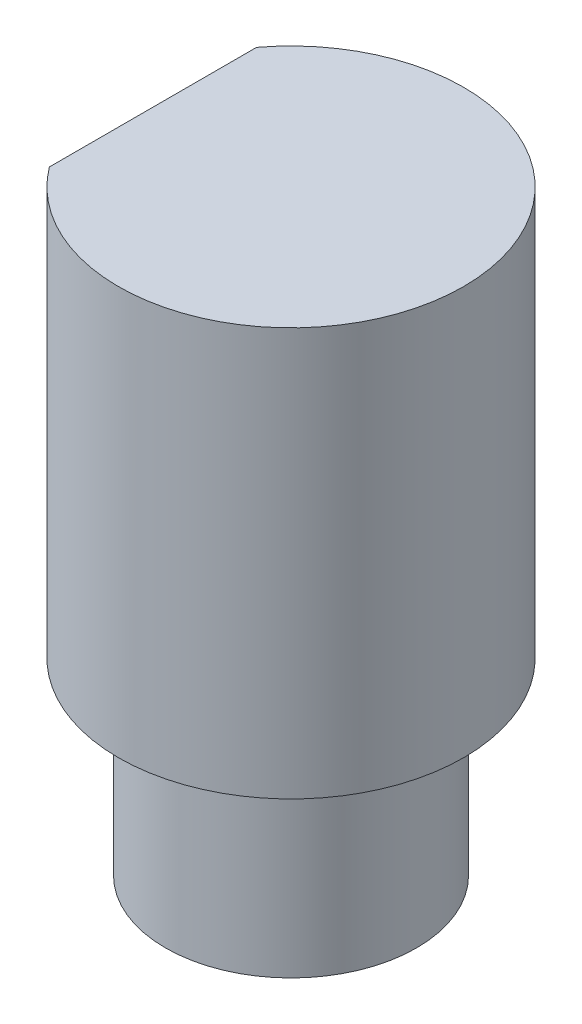
from build123d import *

# Parameters (mm, degrees)
SKETCH1_R           = 20
BOSS_EXTRUDE1_DEPTH = 30
SKETCH2_R           = 27.5
BOSS_EXTRUDE2_DEPTH = 65
CUT_EXTRUDE1_START  = -22
SKETCH3_W           = 35
SKETCH3_H           = 55
CUT_EXTRUDE1_DEPTH  = 65
SKETCH4_R           = 11.3
CUT_EXTRUDE2_DEPTH  = 40
SKETCH5_R           = 9.3
CUT_EXTRUDE3_DEPTH  = 74


with BuildPart() as part:
    # Sketch1 → Boss-Extrude1 (new body)
    with BuildSketch(Plane(origin=(0, 0, 0), x_dir=(1, 0, 0), z_dir=(0, 1, 0))):
        with Locations(Location((0, 0, 0), (0, 0, 270))):
            Circle(SKETCH1_R)
    extrude(amount=BOSS_EXTRUDE1_DEPTH)

    # Sketch2 → Boss-Extrude2 (add)
    with BuildSketch(Plane(origin=(0, 30, 0), x_dir=(1, 0, 0), z_dir=(0, 1, 0))):
        with Locations(Location((0, 0, 0), (0, 0, 270))):
            Circle(SKETCH2_R)
    extrude(amount=BOSS_EXTRUDE2_DEPTH)

    # Sketch3 → Cut-Extrude1 (cut)
    with BuildSketch(Plane(origin=(0, 0, 0), x_dir=(0, 0, -1), z_dir=(1, 0, 0)).offset(CUT_EXTRUDE1_START)):
        with Locations((0, 67.5)):
            Rectangle(SKETCH3_W, SKETCH3_H)
    extrude(amount=-CUT_EXTRUDE1_DEPTH, mode=Mode.SUBTRACT)

    # Sketch4 → Cut-Extrude2 (cut)
    with BuildSketch(Plane.ZY.offset(22)):
        with Locations((0, 73)):
            Circle(SKETCH4_R)
    extrude(amount=-CUT_EXTRUDE2_DEPTH, mode=Mode.SUBTRACT)

    # Sketch5 → Cut-Extrude3 (cut)
    with BuildSketch(Plane.XZ):
        with Locations(Location((0, 0, 0), (0, 0, 270))):
            Circle(SKETCH5_R)
    extrude(amount=-CUT_EXTRUDE3_DEPTH, mode=Mode.SUBTRACT)


solid = part.part
